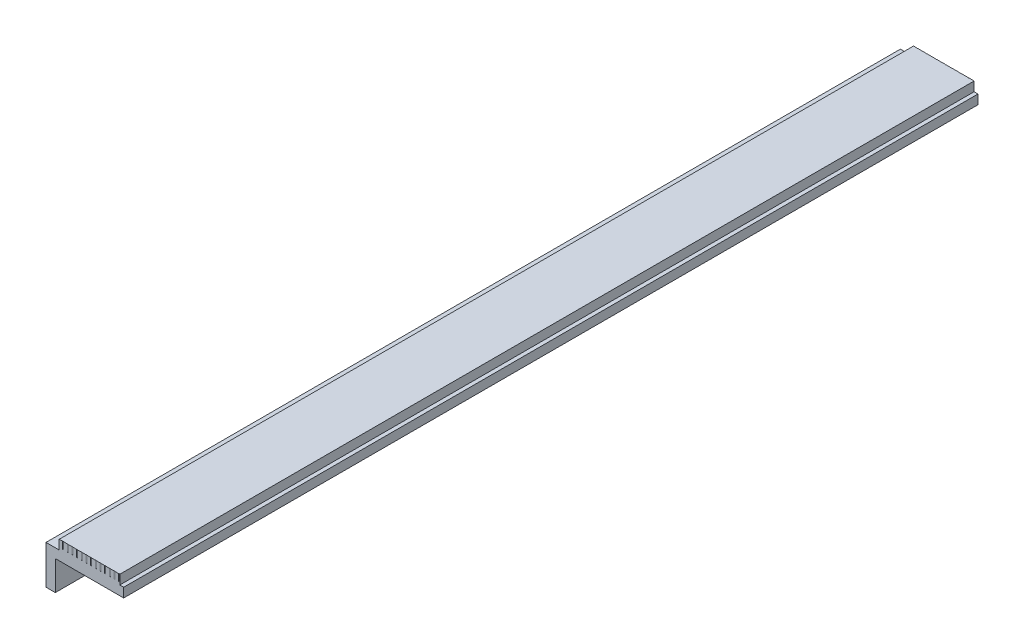
SolidWorks part; units mm, degrees
ref_plane "Front Plane" through (0, 0, 0) normal (0, 0, 1) x (1, 0, 0)
ref_plane "Top Plane" through (0, 0, 0) normal (0, 1, 0) x (1, 0, 0)
ref_plane "Right Plane" through (0, 0, 0) normal (1, 0, 0) x (0, 0, -1)
other "Configuration Table"
sketch "Sketch1" plane through (0, 0, 0) normal (0, 0, 1) x (1, 0, 0)
  line L0 (0, 0) -> (100, 0)
  line L1 (0, 0) -> (0, 100)
  line L2 (12, 12) -> (17, 12)
  line L3 (12, 12) -> (12, 100)
  line L4 (12, 100) -> (0, 100)
  line L5 (100, 12) -> (100, 0)
  line L6 (17, 12) -> (17, 24)
  line L7 (17, 24) -> (95, 24)
  line L8 (95, 24) -> (95, 12)
  line L9 (95, 12) -> (100, 12)
  line L10 (12, 12) -> (100, 12) construction
  dimension "D1" = 100
  dimension "D2" = 100
  dimension "D4" = 12
  dimension "D5" = 5
  dimension "D6" = 5
  dimension "D3" = 12
extrude "Boss-Extrude1" add sketch "Sketch1" along normal blind 1100
sketch "Sketch2" plane through (0, 0, 1100) normal (0, 0, 1) x (1, 0, 0)
  line L0 (95, 24) -> (17, 24) construction
  line L1 (21.4792, 24) -> (22.7391, 24)
  line L2 (21.4792, 24) -> (21.4792, 14.9569)
  line L3 (21.4792, 14.9569) -> (22.7391, 14.9569)
  line L4 (22.7391, 24) -> (22.7391, 14.9569)
  line L5 (21.4792, 24) -> (22.7391, 14.9569) construction
  line L6 (21.4792, 14.9569) -> (22.7391, 24) construction
  point P0 (22.1092, 19.4785)
extrude "Cut-Extrude1" cut sketch "Sketch2" against normal blind 0.2
pattern_linear "LPattern1" count 16 spacing 6 along (1, 0, 0) of "Cut-Extrude1"
ref_plane "Plane1" through (0, 0, 550) normal (0, 0, -1) x (-1, 0, 0)
mirror "Mirror1" about plane through (0, 0, 550) normal (0, 0, -1) of "LPattern1", "Cut-Extrude1"
sketch "Sketch3" plane through (0, 0, 1100) normal (0, 0, 1) x (1, 0, 0)
  line L1 (12, 12) -> (0, 12)
  line L2 (12, 12) -> (12, -38)
  line L3 (12, -38) -> (0, -38)
  line L4 (0, 12) -> (0, -38)
  dimension "D1" = 50
extrude "Boss-Extrude2" add sketch "Sketch3" against normal blind 1100
sketch "Sketch4" plane through (0, 0, 1100) normal (0, 0, 1) x (1, 0, 0)
  line L0 (0, 100) -> (0, -38) construction
  line L1 (12, 100) -> (0, 100)
  line L2 (12, 100) -> (12, 12)
  line L3 (12, 12) -> (0, 12)
  line L4 (0, 100) -> (0, 12)
extrude "Cut-Extrude2" cut sketch "Sketch4" against normal through all
